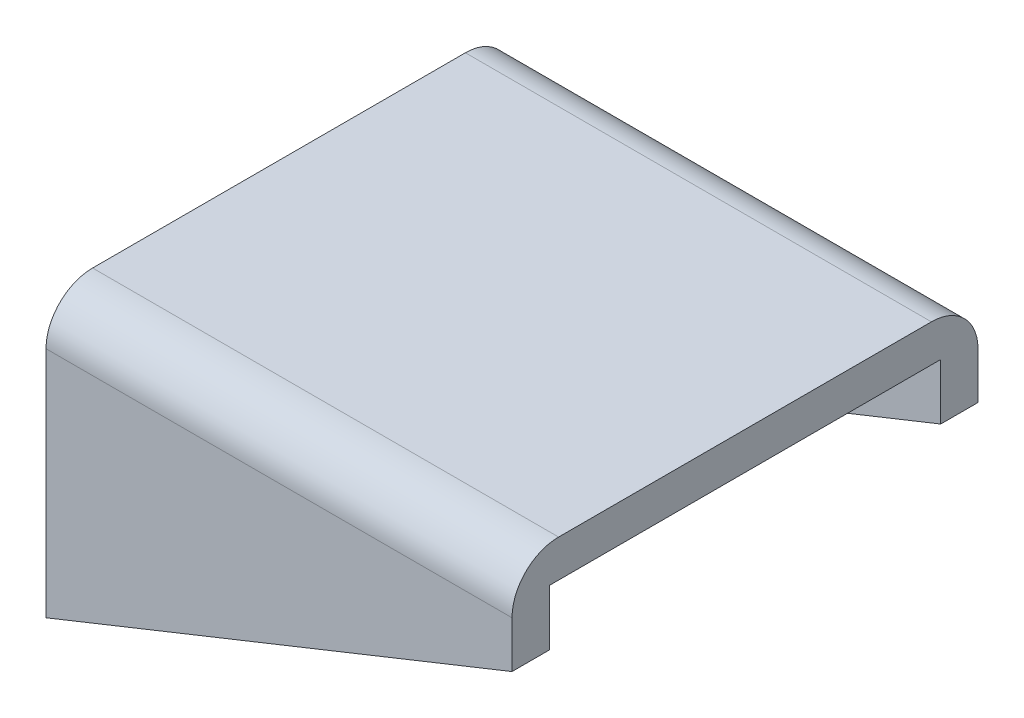
from build123d import *

# Parameters (mm, degrees)
EXTRUDE_1_DEPTH = 100
SHELL_1_T       = -8
FILLET_1_R      = 10
FILLET_2_R      = 10


with BuildPart() as part:
    # 草图1 → 凸台-拉伸1 (new body)
    with BuildSketch(Plane.XY):
        Polygon((0, 0), (0, 60), (100, 60), (100, 40), align=None)
    extrude(amount=EXTRUDE_1_DEPTH)

    # 抽壳1
    shell_1_openings = [part.faces().sort_by_distance(p)[0] for p in [
        (0, 30, 50),
        (100, 50, 50),
        (50, 20, 50),
    ]]
    offset(amount=SHELL_1_T, openings=shell_1_openings, kind=Kind.INTERSECTION)

    # 圆角1
    fillet_1_edges = [part.edges().sort_by_distance(p)[0] for p in [
        (50, 60, 100),
    ]]
    fillet(fillet_1_edges, radius=FILLET_1_R)

    # 圆角2
    fillet_2_edges = [part.edges().sort_by_distance(p)[0] for p in [
        (50, 60, 0),
    ]]
    fillet(fillet_2_edges, radius=FILLET_2_R)


solid = part.part
